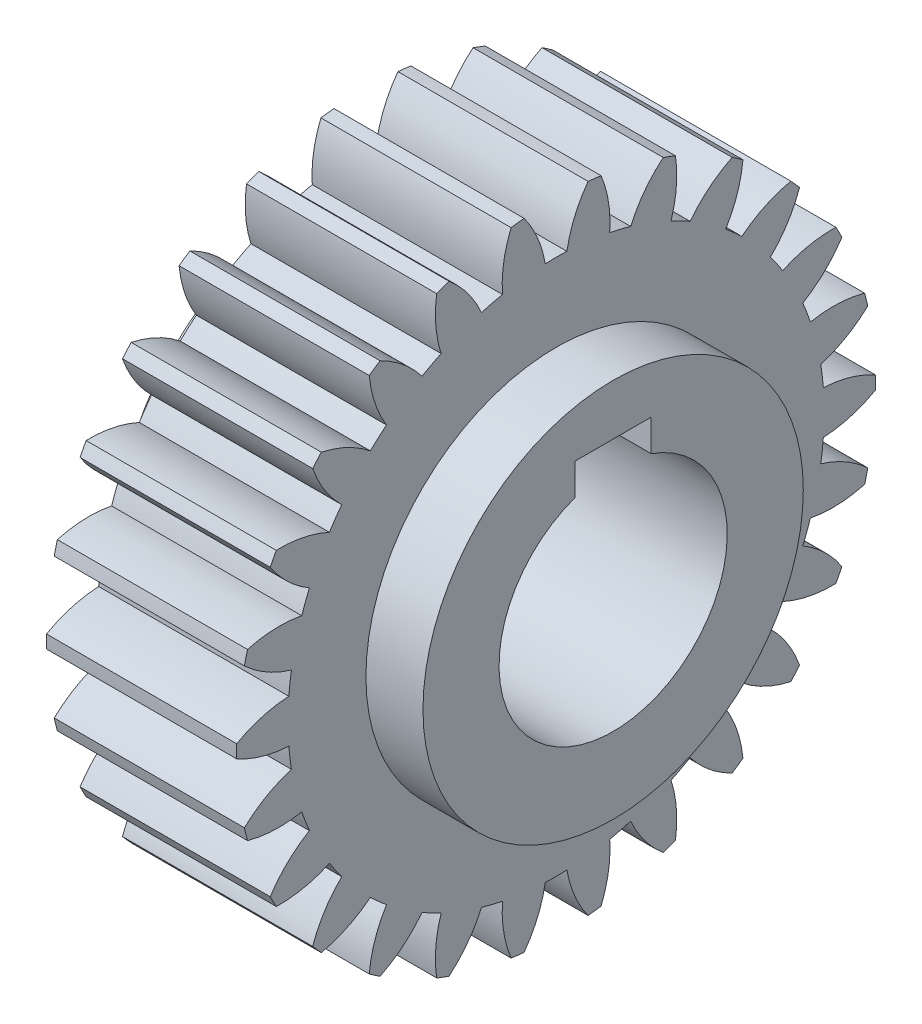
SolidWorks part; units mm, degrees
ref_plane "Plane1" through (0, 0, 0) normal (0, 0, 1) x (1, 0, 0)
ref_plane "Plane2" through (0, 0, 0) normal (0, 1, 0) x (1, 0, 0)
ref_plane "Plane3" through (0, 0, 0) normal (1, 0, 0) x (0, 0, -1)
sketch "HoldingSke" plane through (0, 0, 0) normal (0, 1, 0) x (1, 0, 0)
  line L0 (0, 0) -> (0.2996, -0.1461)
  line L1 (-15, 0) -> (100, 0) construction
  line L2 (0, 0) -> (-2.1039, 2.3779)
  line L3 (0, 0) -> (-11.863, 4.5341)
  line L4 (0, 0) -> (7.762, 3.7858)
  line L5 (0, 0) -> (-37.4781, -13.9782)
  line L6 (0, 0) -> (-20.7241, -13.9826)
  line L7 (-2.1039, 2.3779) -> (6.5061, 41.4403)
  line L8 (-76.2, 54.61) -> (-72.9, 54.61)
  line L9 (-71.009, 38.7566) -> (-53.1078, 45.2721)
  line L10 (-76.2, 71.12) -> (104.1128, 71.12)
  line L11 (0, 0) -> (-25, 0)
  line L12 (-76.2, 101.6) -> (-76.093, 101.6)
  line L13 (24.9733, 27.94) -> (52.9518, 28.4284)
  line L14 (24.9733, 27.94) -> (24.9743, 27.94)
  line L15 (24.9733, 27.94) -> (100.4006, 29.5858)
  line L16 (-63.627, -3) -> (-12.827, -3)
  circle A0 centre (0, 0) radius 15
  circle A1 centre (0, 0) radius 25
  circle A2 centre (0, 0) radius 25
  circle A3 centre (0, 0) radius 15
sketch "BasProSke" plane through (0, 0, 0) normal (0, 1, 0) x (1, 0, 0)
  line L0 (-10, 0) -> (60, 0) construction
  line L1 (0, 0) -> (0, 42)
  line L2 (0, 0) -> (25, 0)
  line L3 (25, 0) -> (25, 42)
  line L4 (25, 42) -> (0, 42)
revolve "Base-Revolve" add sketch "BasProSke" angle 360 about L0
sketch "TooCutSke" plane through (0, 0, 0) normal (1, 0, 0) x (0, 0, -1)
  line L1 (0, 0) -> (0, 107) construction
  line L2 (0, 0) -> (-2.542, 38.9171) construction
  line L3 (0, 0) -> (-9.3873, 77.3116) construction
  line L4 (-2.542, 38.9171) -> (-4.6937, 38.6558) construction
  arc A0 (1.4202, 35.2204) -> (-1.4202, 35.2204) centre (0, 0) ccw
  arc A1 (4.2241, 41.8126) -> (-4.2241, 41.8126) centre (0, 0) ccw
  circle A2 centre (0, 0) radius 39 construction
  circle A3 centre (0, 0) radius 36.648 construction
  arc A4 (-1.4202, 35.2204) -> (-4.2241, 41.8126) centre (-16.794, 32.5736) ccw
  arc A5 (4.2241, 41.8126) -> (1.4202, 35.2204) centre (16.794, 32.5736) ccw
extrude "ToothCut" cut sketch "TooCutSke" along normal through all
fillet "Breaks" [suppressed] radius 0.06
fillet "RootFillets" [suppressed] radius 0.751
pattern_circular "TeethCuts" count 26 every 13.846 about axis through (-10, 0, 0) along (1, 0, 0) of "ToothCut", "RootFillets", "Breaks"
sketch "HubNeaOneSke" plane through (0, 0, 0) normal (-1, 0, 0) x (0, 0, 1)
  circle A0 centre (0, 0) radius 25
extrude "HubNearOne" [suppressed] add sketch "HubNeaOneSke" along normal blind 15.0001
sketch "HubNeaBotSke" plane through (0, 0, 0) normal (-1, 0, 0) x (0, 0, 1)
  circle A0 centre (0, 0) radius 25
extrude "HubNearBoth" add sketch "HubNeaBotSke" along normal blind 7.5
ref_plane "FarPln" through (25, 0, 0) normal (1, 0, 0) x (0, 0, -1)
sketch "HubFarSke" plane through (25, 0, 0) normal (1, 0, 0) x (0, 0, -1)
  circle A0 centre (0, 0) radius 25
extrude "HubFar" add sketch "HubFarSke" along normal blind 7.5
sketch "BorSke" plane through (0, 0, 0) normal (1, 0, 0) x (0, 0, -1)
  circle A0 centre (0, 0) radius 15
extrude "Bore" cut sketch "BorSke" along normal mid plane 80.0001
sketch "KeySke" plane through (0, 0, 0) normal (1, 0, 0) x (0, 0, -1)
  line L0 (-5, 0) -> (-5, 18.3)
  line L1 (-5, 18.3) -> (5, 18.3)
  line L2 (5, 18.3) -> (5, 0)
  line L3 (0, 0) -> (0, 34) construction
  line L4 (-5, 0) -> (5, 0)
extrude "Keyway" cut sketch "KeySke" along normal mid plane 80.0001
pattern_circular "Keyway2" [suppressed] count 2 every 90 about axis through (-10, 0, 0) along (1, 0, 0)
equation "' \"Module@HoldingSke\" = 6.35"
equation "' \"Num_teeth@HoldingSke\" = 12"
equation "' \"Ap@HoldingSke\" =  20"
equation "' \"Ap@HoldingSke\" = 20"
equation "' \"Width@HoldingSke\" = 0.5 * 25.4"
equation "' \"Hub_dia@HoldingSke\"= 1 * 25.4"
equation "' \"Hub_dia@HoldingSke\" = 1 * 25.4"
equation "' \"Overall_len@HoldingSke\" = 1.0 * 25.4"
equation "' \"Bore@HoldingSke\" = 0.75 * 25.4"
equation "' \"T_dim@HoldingSke\" = 0.1 * 25.4"
equation "' \"Width@KeySke\" = 0.25 * 25.4"
equation "' \"Show_teeth@HoldingSke\" = 13"
equation "' \"Backlash@HoldingSke\" = 0.009 * 25.4"
equation "' \"Addendum_fac@HoldingSke\" = 1.0"
equation "' \"Dedendum_fac@HoldingSke\" = 1.25"
equation "' \"Dedendum_add@HoldingSke\" = 0.00005 * 25.4"
equation "' \"Clearance_fac@HoldingSke\" = 0.25"
equation "\"Pitch@HoldingSke\" = 1 / \"Module@HoldingSke\""
equation "\"Overcut_dia@TooCutSke\" = (\"Num_teeth@HoldingSke\" + 2 * \"Addendum_fac@HoldingSke\") / \"Pitch@HoldingSke\" + 0.002 * 25.4"
equation "\"Pitch_dia@TooCutSke\" = \"Num_teeth@HoldingSke\" / \"Pitch@HoldingSke\""
equation "\"Base_dia@TooCutSke\" = \"Num_teeth@HoldingSke\" / \"Pitch@HoldingSke\" * cos((\"Ap@HoldingSke\"  * 3.14159265 / 180))"
equation "\"Root_dia@TooCutSke\" = (\"Num_teeth@HoldingSke\" + 2) / \"Pitch@HoldingSke\" - 2 * (\"Addendum_fac@HoldingSke\" + \"Dedendum_fac@HoldingSke\") / \"Pitch@HoldingSke\" - \"Dedendum_add@HoldingSke\" * 2"
equation "\"Half_ang@TooCutSke\" = 180 / \"Num_teeth@HoldingSke\""
equation "\"Half_CT@TooCutSke\" = \"Num_teeth@HoldingSke\" / \"Pitch@HoldingSke\" * sin((3.14159265 / 2 / \"Num_teeth@HoldingSke\")) / 2 - 7 * \"Backlash@HoldingSke\" / 4"
equation "\"Flank_rad@TooCutSke\" = \"Num_teeth@HoldingSke\" / \"Pitch@HoldingSke\" / 5"
equation "\"Radius@RootFillets\" = \"Clearance_fac@HoldingSke\" / \"Pitch@HoldingSke\" + \"Dedendum_add@HoldingSke\""
equation "\"Break_rad@Breaks\" = 0.02 / \"Pitch@HoldingSke\""
equation "\"Thickness@HoldingSke\" = \"Width@HoldingSke\""
equation "\"OAL@HoldingSke\" = \"Thickness@HoldingSke\""
equation "\"MHD@HoldingSke\" = (\"Num_teeth@HoldingSke\" + 2) / \"Pitch@HoldingSke\" - 2 * (\"Addendum_fac@HoldingSke\" + \"Dedendum_fac@HoldingSke\")  / \"Pitch@HoldingSke\" - \"Dedendum_add@HoldingSke\" * 2"
equation "\"MBD@HoldingSke\" = (\"Num_teeth@HoldingSke\" + 2) / \"Pitch@HoldingSke\" - 2 * (\"Addendum_fac@HoldingSke\" + \"Dedendum_fac@HoldingSke\")  / \"Pitch@HoldingSke\" - \"Dedendum_add@HoldingSke\" * 2 - 0.002 * 25.4"
equation "\"MHD@HoldingSke\" = ((sgn( \"MHD@HoldingSke\" - \"Hub_dia@HoldingSke\" )-1)*( \"MHD@HoldingSke\" - \"Hub_dia@HoldingSke\" ))/-2+ \"Hub_dia@HoldingSke\""
equation "\"MBD@HoldingSke\" = ((sgn( \"MBD@HoldingSke\" - \"Bore@HoldingSke\" )-1)*( \"MBD@HoldingSke\" - \"Bore@HoldingSke\" ))/-2+ \"Bore@HoldingSke\""
equation "\"OAL@HoldingSke\" = ((sgn( \"OAL@HoldingSke\" - \"Overall_len@HoldingSke\" )+1)*( \"OAL@HoldingSke\" - \"Overall_len@HoldingSke\" ))/2 + \"Overall_len@HoldingSke\" + 0.000002 * 25.4"
equation "\"Num_teeth@TeethCuts\" = int( \"Show_teeth@HoldingSke\" ) + 1"
equation "\"Num_teeth@TeethCuts\" = ((sgn( \"Num_teeth@TeethCuts\" - \"Num_teeth@HoldingSke\" )-1)*( \"Num_teeth@TeethCuts\" - \"Num_teeth@HoldingSke\" ))/-2+ \"Num_teeth@HoldingSke\""
equation "\"Num_teeth@TeethCuts\" = ((sgn( \"Num_teeth@TeethCuts\" - 2.0)+1)*( \"Num_teeth@TeethCuts\" - 2.0))/2 +2.0"
equation "\"Angle@TeethCuts\" = 360.0 / \"Num_teeth@HoldingSke\""
equation "\"Diameter@BasProSke\" = (\"Num_teeth@HoldingSke\" + 2 * \"Addendum_fac@HoldingSke\") / \"Pitch@HoldingSke\""
equation "\"Thickness@BasProSke\"  = \"Thickness@HoldingSke\""
equation "' \"Fillet_rad@BasProSke\" =  \"Thickness@HoldingSke\" * 0.05"
equation "' \"Fillet_rad@BasProSke\" = \"Thickness@HoldingSke\" * 0.05"
equation "\"MHD@HoldingSke\" = ((sgn( \"MHD@HoldingSke\" - \"Root_dia@TooCutSke\" )-1)*( \"MHD@HoldingSke\" - \"Root_dia@TooCutSke\" ))/-2+ \"Root_dia@TooCutSke\""
equation "\"Diameter@HubNeaOneSke\" = \"MHD@HoldingSke\""
equation "\"Length@HubNearOne\" = \"OAL@HoldingSke\" - \"Thickness@BasProSke\""
equation "\"Diameter@HubNeaBotSke\" = \"MHD@HoldingSke\""
equation "\"Length@HubNearBoth\" = ( \"OAL@HoldingSke\" - \"Thickness@BasProSke\" ) / 2.0"
equation "\"Thickness@FarPln\" = \"Thickness@BasProSke\""
equation "\"Diameter@HubFarSke\" = \"MHD@HoldingSke\""
equation "\"Length@HubFar\" = ( \"OAL@HoldingSke\" - \"Thickness@BasProSke\" ) / 2.0"
equation "\"Diameter@BorSke\" = \"MBD@HoldingSke\""
equation "\"D1@Bore\" = \"OAL@HoldingSke\" * 2.0"
equation "\"D1@Keyway\" = \"OAL@HoldingSke\" * 2.0"
equation "\"Offset@KeySke\" = \"T_dim@HoldingSke\" + \"MBD@HoldingSke\" / 2.0"
